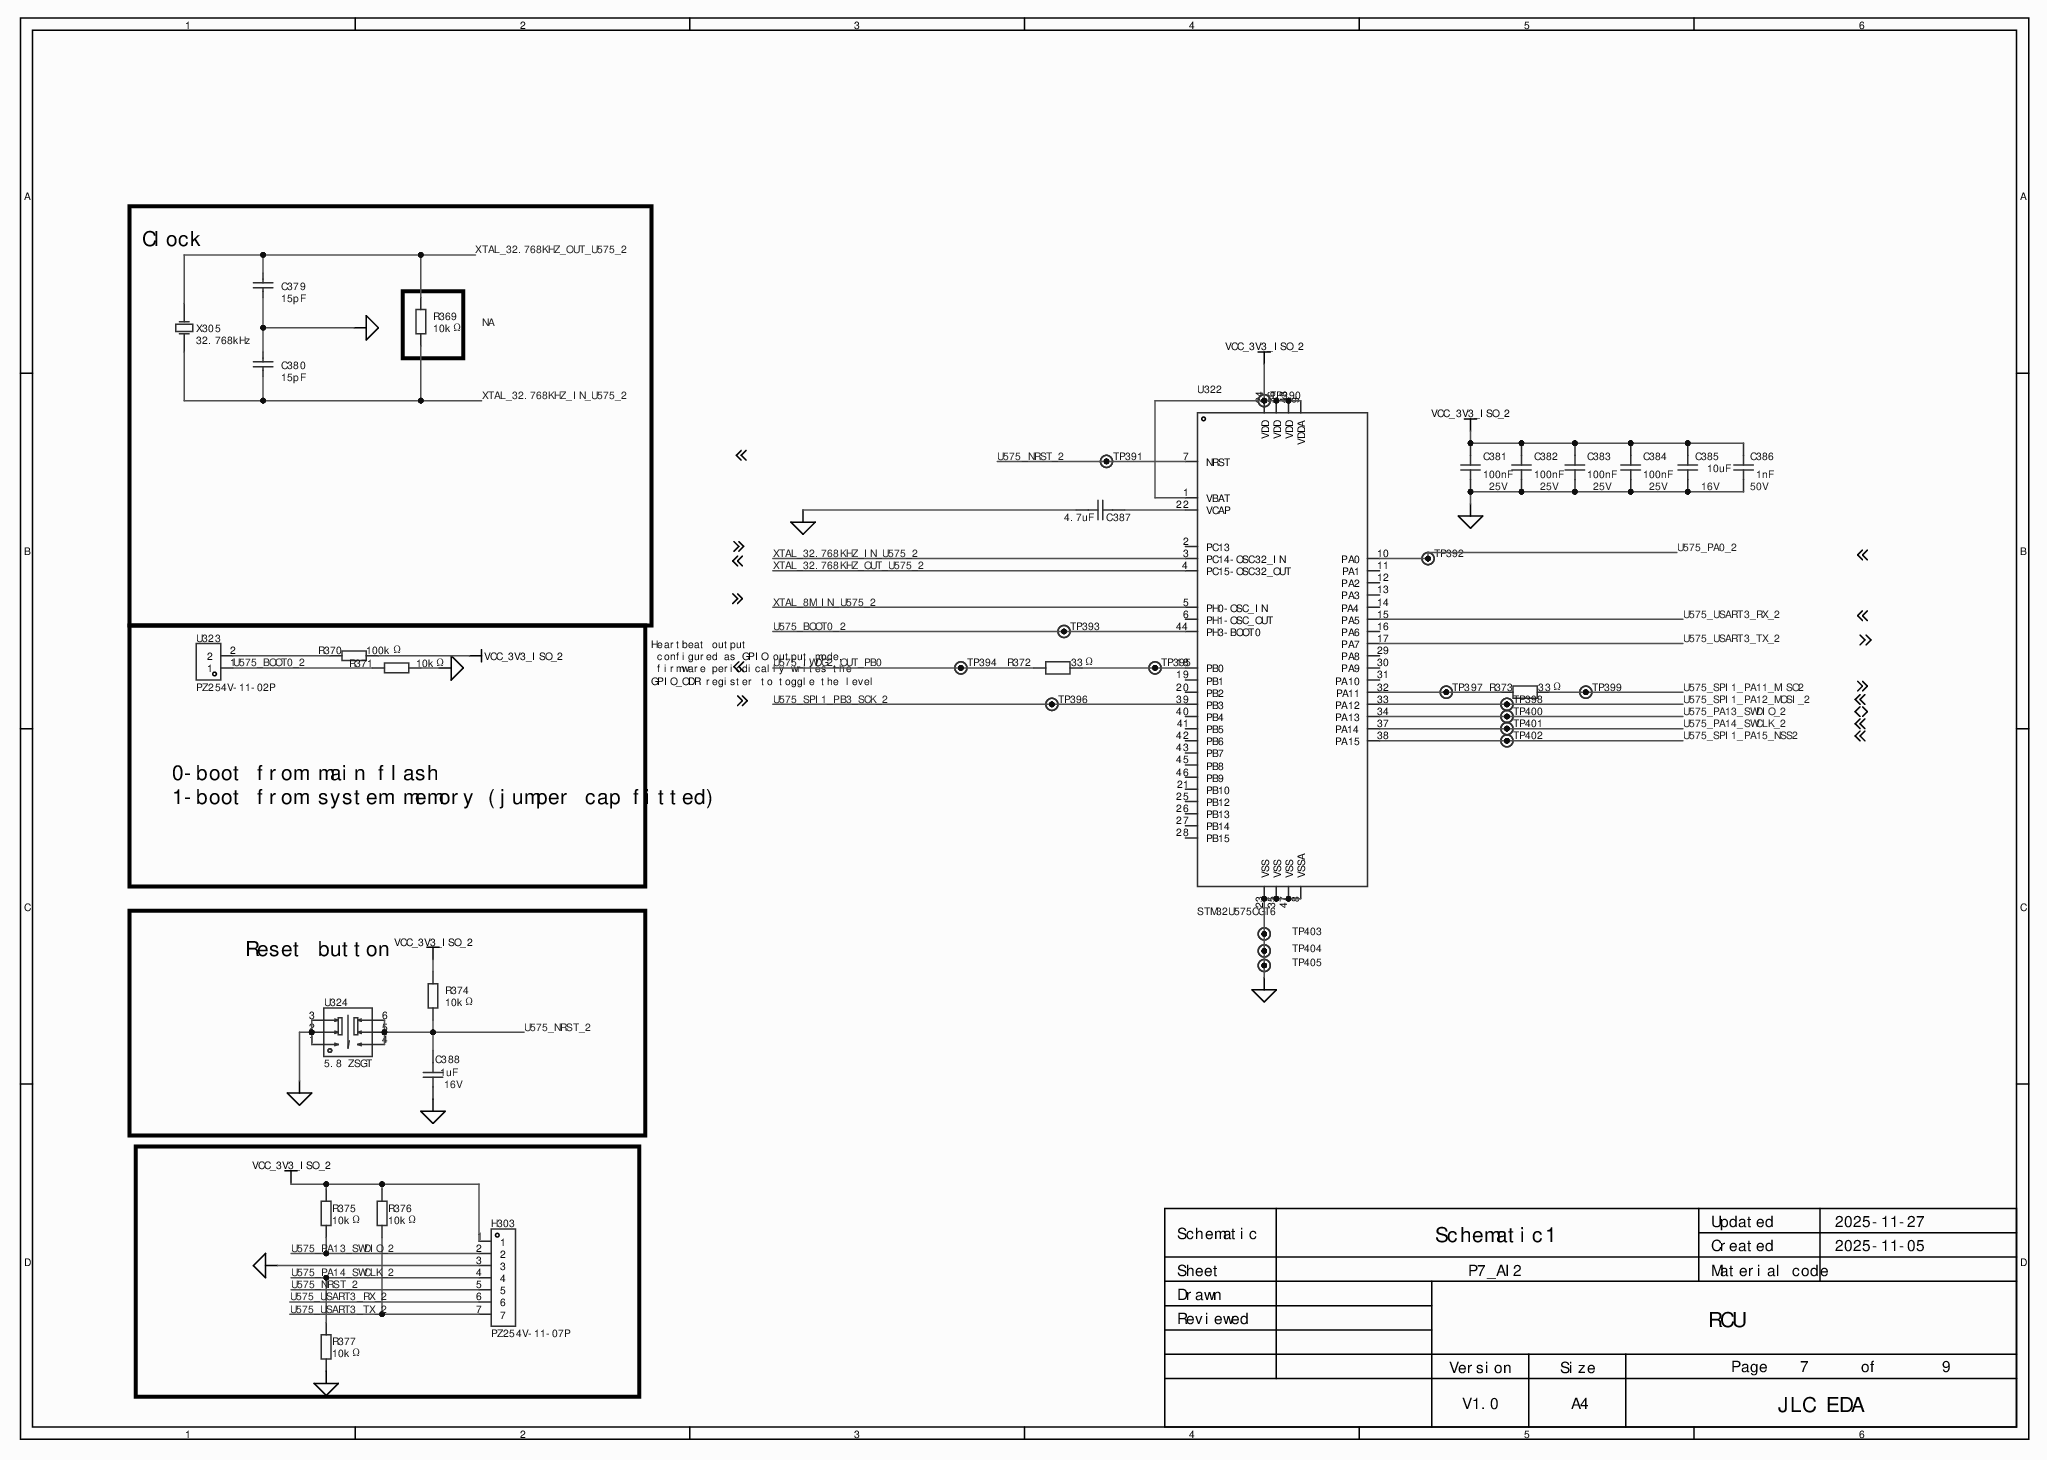
[diagram p0: MISC84429-8.SchDoc]
# Altium project MISC84429-12.PrjPcb (part 4 of 5)

## Sheet MISC84429-8.SchDoc
size 431 x 309 mm; Name: Sheet-Symbol; Symbol: Sheet-Symbol; Device: Sheet-Symbol

### Parts
C379  15pF  [C0402]
C380  15pF  [C0402]
C381  100nF  Voltage Rated: 25V  [C0603]
C382  100nF  Voltage Rated: 25V  [C0603]
C383  100nF  Voltage Rated: 25V  [C0603]
C384  100nF  Voltage Rated: 25V  [C0603]
C385  10uF  Voltage Rated: 16V  [C0805]
C386  1nF  Voltage Rated: 50V  [C0603]
C387  4.7uF  [C0603]
C388  1uF  Voltage Rated: 16V  [C0603]
H303  PZ254V-11-07P  [HDR-TH_7P-P2.54-V-M]
R369  10kΩ  [R0402]
R370  100kΩ  [R0603]
R371  10kΩ  [R0603]
R372  33Ω  [R0603]
R373  33Ω  [R0603]
R374  10kΩ  [R0402]
R375  10kΩ  [R0603]
R376  10kΩ  [R0603]
R377  10kΩ  [R0603]
TP390  (no value)  [Test-Point-0.5mm]
TP391  (no value)  [Test-Point-0.5mm]
TP392  (no value)  [Test-Point-0.5mm]
TP393  (no value)  [Test-Point-0.5mm]
TP394  (no value)  [Test-Point-0.5mm]
TP395  (no value)  [Test-Point-0.5mm]
TP396  (no value)  [Test-Point-0.5mm]
TP397  (no value)  [Test-Point-0.5mm]
TP398  (no value)  [Test-Point-0.5mm]
TP399  (no value)  [Test-Point-0.5mm]
TP400  (no value)  [Test-Point-0.5mm]
TP401  (no value)  [Test-Point-0.5mm]
TP402  (no value)  [Test-Point-0.5mm]
TP403  (no value)  [Test-Point-0.5mm]
TP404  (no value)  [Test-Point-0.5mm]
TP405  (no value)  [Test-Point-0.5mm]
U322  STM32U575CGT6  [LQFP-48_L7.0-W7.0-P0.50-LS9.0-TL]
U323  PZ254V-11-02P  [HDR-TH_2P-P2.54-V-M]
U324  5.8 ZSGT  [SW-TH_5.8ZSGT]
X305  32.768kHz  [OSC-TH_BD3.1-P0.8-D0.3]

### Blocks framed on the sheet
Clock: C379 C380 R369 X305
Reset button: C388 R374 U324

### Nets
PGND: C379.1 C380.2 C381.2 C382.2 C383.2 C384.2 C385.1 C386.1 C387.2 C388.1 H303.3 R371.1 R377.2 TP403.1 TP404.1 TP405.1 U322.8(VSSA) U322.23(VSS) U322.35(VSS) U322.47(VSS) U324.1 U324.2 U324.3
VCC_3V3_ISO_2: C381.1 C382.1 C383.1 C384.1 C385.2 C386.2 H303.1 R370.2 R374.2 R375.2 R376.2 TP390.1 U322.1(VBAT) U322.9(VDDA) U322.24(VDD) U322.36(VDD) U322.48(VDD)
U575_BOOT0_2: R371.2 TP393.1 U322.44(PH3-BOOT0) U323.1
U575_IWDG2_OUT_PB0: R372.2 TP394.1
U575_NRST_2: C388.2 H303.5 R374.1 TP391.1 U322.7(NRST) U324.4 U324.5 U324.6
U575_PA0_2: TP392.1 U322.10(PA0)
U575_PA13_SWDIO_2: H303.2 R375.1 TP400.1 U322.34(PA13)
U575_PA14_SWCLK_2: H303.4 R377.1 TP401.1 U322.37(PA14)
U575_SPI1_PA11_MISO2: R373.1 TP399.1
U575_SPI1_PA12_MOSI_2: TP398.1 U322.33(PA12)
U575_SPI1_PA15_NSS2: TP402.1 U322.38(PA15)
U575_SPI1_PB3_SCK_2: TP396.1 U322.39(PB3)
U575_USART3_RX_2: H303.6 U322.15(PA5)
U575_USART3_TX_2: H303.7 R376.1 U322.17(PA7)
XTAL_8M_IN_U575_2: U322.5(PH0-OSC_IN)
XTAL_32.768KHZ_IN_U575_2: C380.1 R369.1 U322.3(PC14-OSC32_IN) X305.1(OSC1)
XTAL_32.768KHZ_OUT_U575_2: C379.2 R369.2 U322.4(PC15-OSC32_OUT) X305.2(OSC2)
NetC387_1: C387.1 U322.22(VCAP)
NetR370_1: R370.1 U323.2
NetR372_1: R372.1 TP395.1 U322.18(PB0)
NetR373_2: R373.2 TP397.1 U322.32(PA11)

Not connected (* = marked no-connect by the designer): U322 2(PC13)* 6(PH1-OSC_OUT)* 11(PA1)* 12(PA2)* 13(PA3)* 14(PA4)* 16(PA6)* 19(PB1)* 20(PB2)* 21(PB10)* 25(PB12)* 26(PB13)* 27(PB14)* 28(PB15)* 29(PA8)* 30(PA9)* 31(PA10)* 40(PB4)* 41(PB5)* 42(PB6)* 43(PB7)* 45(PB8)* 46(PB9)*

### Notes on the sheet
- NA
- Heartbeat output
  configured as GPIO output mode,
  firmware periodically writes the
  GPIO_ODR register to toggle the level
- 0-boot from main flash
  1-boot from system memory (jumper cap fitted)
- 1
- 2
- 3
- 4
- 5
- 6
- A
- B
- C
- D
- Schematic
- Schematic1
- Created
- Updated
- 2025-11-27
- 2025-11-05
- Reviewed
- Drawn
- Sheet
- P7_AI2
- Material code
- RCU
- Version
- Size
- Page
- 7
- of
- 9
- V1.0
- A4
- JLC EDA

### Library data of the parts
C379 C380 = GJM1555C1H150FB01D: Manufacturer: muRata(村田); Add into BOM: yes; Tolerance: ±1%; Voltage Rated: 50V; Temperature Coefficient: C0G; Symbol: GJM1555C1H150FB01D; Device: GJM1555C1H150FB01D; LCSC Part Name: 15pF ±1% 50V; Supplier Part: C441742; Manufacturer Part: GJM1555C1H150FB01D; Supplier Footprint: 0402; JLCPCB Part Class: Extended library; Datasheet: https://atta.szlcsc.com/upload/public/pdf/source/20200305/C490387_23319AE8C154DEB24C505E6C82A8106A.pdf; Supplier: LCSC; Convert to PCB: yes; Value: 15pF; Origin Footprint: C0402
C381-C384 = GRM188R71E104KA01D: Manufacturer: muRata(村田); Add into BOM: yes; Tolerance: ±10%; Temperature Coefficient: X7R; Symbol: GRM188R71E104KA01D; Device: GRM188R71E104KA01D; LCSC Part Name: 100nF ±10% 25V; Supplier Part: C77050; Manufacturer Part: GRM188R71E104KA01D; Supplier Footprint: 0603; JLCPCB Part Class: Extended library; Datasheet: https://atta.szlcsc.com/upload/public/pdf/source/20170622/1498103881034.pdf; Supplier: LCSC; Convert to PCB: yes; Value: 100nF; Origin Footprint: C0603
C385 = GRM21BR61C106KE15L: Manufacturer: muRata(村田); Add into BOM: yes; Tolerance: ±10%; Temperature Coefficient: X5R; Symbol: GRM21BR61C106KE15L; Device: GRM21BR61C106KE15L; LCSC Part Name: 10uF ±10% 16V; Supplier Part: C77075; Manufacturer Part: GRM21BR61C106KE15L; Supplier Footprint: 0805; JLCPCB Part Class: Extended library; Datasheet: https://atta.szlcsc.com/upload/public/pdf/source/20200305/C490387_23319AE8C154DEB24C505E6C82A8106A.pdf; Supplier: LCSC; Convert to PCB: yes; Value: 10uF; Origin Footprint: C0805
C386 = GRM1885C1H102JA01D: Manufacturer: muRata(村田); Add into BOM: yes; Tolerance: ±5%; Temperature Coefficient: C0G; Symbol: GRM1885C1H102JA01D; Device: GRM1885C1H102JA01D; LCSC Part Name: 1nF ±5% 50V; Supplier Part: C77026; Manufacturer Part: GRM1885C1H102JA01D; Supplier Footprint: 0603; JLCPCB Part Class: Extended library; Datasheet: https://atta.szlcsc.com/upload/public/pdf/source/20200305/C490387_23319AE8C154DEB24C505E6C82A8106A.pdf; Supplier: LCSC; Convert to PCB: yes; Value: 1nF; Origin Footprint: C0603
C387 = GRT188C81E475KE13D: Manufacturer: muRata(村田); Add into BOM: yes; Tolerance: ±10%; Voltage Rating: 25V; Temperature Coefficient: X6S; Symbol: GRT188C81E475KE13D; Device: GRT188C81E475KE13D; LCSC Part Name: 4.7uF ±10% 25V; Supplier Part: C907917; Manufacturer Part: GRT188C81E475KE13D; Supplier Footprint: 0603; JLCPCB Part Class: Extended library; Datasheet: https://item.szlcsc.com/datasheet/GRT188C81E475KE13D/973818.html; Supplier: LCSC; Convert to PCB: yes; Value: 4.7uF; Origin Footprint: C0603
C388 = GCM188R71C105KA64D: Manufacturer: muRata(村田); Add into BOM: yes; Tolerance: ±10%; Temperature Coefficient: X7R; Symbol: GCM188R71C105KA64D; Device: GCM188R71C105KA64D; LCSC Part Name: 1uF ±10% 16V; Supplier Part: C161212; Manufacturer Part: GCM188R71C105KA64D; Supplier Footprint: 0603; JLCPCB Part Class: Extended library; Datasheet: https://atta.szlcsc.com/upload/public/pdf/source/20181221/C161212_C96DD77354D5551432B3B7779E4D1948.pdf; Supplier: LCSC; Convert to PCB: yes; Value: 1uF; Origin Footprint: C0603
H303 = PZ254V-11-07P: Manufacturer: XFCN(兴飞); Add into BOM: yes; Pin Structure: 1x7P; Pitch: 2.54mm; Circluar Pins/Square Pins: Square pin; Symbol: PZ254V-11-07P; Device: PZ254V-11-07P; LCSC Part Name: 1x7P 间距:2.54mm 方针 直插; Supplier Part: C492406; Manufacturer Part: PZ254V-11-07P; Supplier Footprint: 插件,P=2.54mm; JLCPCB Part Class: Extended library; Datasheet: https://atta.szlcsc.com/upload/public/pdf/source/20200309/C492406_654C533EE691117E22DD9F76C114C2D9.pdf; Supplier: LCSC; Convert to PCB: yes; Row Spacing: -; Mounting Type: Through hole; Number of Rows: Single row; Number of Pins: 7P; Current Rating: -; Voltage Rating (Max): -; Length of Mating Pin: 6mm; Insulation Height: 2.5mm; Length of End Connection Pin: 3mm; Contact Material: Brass; Contact Plating: -; Operating Temperature: -40℃~+105℃; Color: Black; Origin Footprint: HDR-TH_7P-P2.54-V-M
R369 R374 = 0402WGF1002TCE: Manufacturer: UNI-ROYAL(厚声); Add into BOM: yes; Tolerance: ±1%; Power(Watts): 62.5mW; Overload Voltage (Max): 50V; Temperature Coefficient: ±100ppm/℃; Symbol: 0402WGF1002TCE; Device: 0402WGF1002TCE; LCSC Part Name: 10kΩ ±1% 62.5mW 厚膜电阻; Supplier Part: C25744; Manufacturer Part: 0402WGF1002TCE; Supplier Footprint: 0402; JLCPCB Part Class: Basic library; Datasheet: https://atta.szlcsc.com/upload/public/pdf/source/20200306/C422600_1E6D84923E4A46A82E41ADD87F860B5C.pdf; Supplier: LCSC; Convert to PCB: yes; Type: Thick film resistor; Value: 10kΩ; Operating Temperature Range: -55℃~+155℃; Origin Footprint: R0402
R370 = RC0603FR-07100KL: Manufacturer: YAGEO(国巨); Add into BOM: yes; Tolerance: ±1%; Power(Watts): 100mW; Overload Voltage (Max): 75V; Temperature Coefficient: ±100ppm/℃; Symbol: RC0603FR-07100KL; Device: RC0603FR-07100KL; LCSC Part Name: 厚膜电阻 100kΩ ±1% 100mW; Supplier Part: C14675; Manufacturer Part: RC0603FR-07100KL; Supplier Footprint: 0603; JLCPCB Part Class: Extended library; Datasheet: https://atta.szlcsc.com/upload/public/pdf/source/20140324/1457707028752.pdf; Supplier: LCSC; Convert to PCB: yes; Type: Thick film resistor; Value: 100kΩ; Operating Temperature Range: -55℃~+155℃; Origin Footprint: R0603
R371 R375-R377 = RC0603FR-0710KL: Manufacturer: YAGEO(国巨); Add into BOM: yes; Tolerance: ±1%; Power(Watts): 100mW; Overload Voltage (Max): 75V; Temperature Coefficient: ±100ppm/℃; Symbol: RC0603FR-0710KL; Device: RC0603FR-0710KL; LCSC Part Name: 厚膜电阻 10kΩ ±1% 100mW; Supplier Part: C98220; Manufacturer Part: RC0603FR-0710KL; Supplier Footprint: 0603; JLCPCB Part Class: Extended library; Datasheet: https://atta.szlcsc.com/upload/public/pdf/source/20180927/C295883_E8D83085EA81BD7DE0B2B681138C15EE.pdf; Supplier: LCSC; Convert to PCB: yes; Type: Thick film resistor; Value: 10kΩ; Operating Temperature Range: -55℃~+155℃; Origin Footprint: R0603
R372 R373 = FRC0603F33R0TS: Manufacturer: FOJAN(富捷); Add into BOM: yes; Tolerance: ±1%; Power(Watts): 100mW; Voltage-Supply(Max): 75V; Temperature Coefficient: ±100ppm/℃; Symbol: FRC0603F33R0TS; Device: FRC0603F33R0TS; LCSC Part Name: 33Ω ±1% 100mW 厚膜电阻; Supplier Part: C2909394; Manufacturer Part: FRC0603F33R0TS; Supplier Footprint: 0603; JLCPCB Part Class: Extended library; Supplier: LCSC; Convert to PCB: yes; Type: Thick film resistor; Value: 33Ω; Operating Temperature: -55℃~+155℃; Origin Footprint: R0603
TP390-TP405 = Test-Point: Add into BOM: yes; Symbol: Test-Point; Device: Test-Point; Convert to PCB: yes; Origin Footprint: Test-Point-0.5mm
U322 = STM32U575CGT6: Manufacturer: ST(意法半导体); Add into BOM: yes; Symbol: STM32U575CGT6; Device: STM32U575CGT6; LCSC Part Name: 超低功耗带 FPU 的 Arm Cortex-M33 具有 Trust Zone，160 MHz MCU 带 1MB 闪存; Supplier Part: C5271006; Manufacturer Part: STM32U575CGT6; Supplier Footprint: LQFP-48(7x7); JLCPCB Part Class: Extended library; Datasheet: https://atta.szlcsc.com/upload/public/pdf/source/20250311/118E46867C2F8A0EF1AEA9206C957AC0.pdf; Supplier: LCSC; Convert to PCB: yes; Origin Footprint: LQFP-48_L7.0-W7.0-P0.50-LS9.0-TL
U323 = PZ254V-11-02P: Manufacturer: XFCN(兴飞); Add into BOM: yes; Pin Structure: 1x2P; Pitch: 2.54mm; Circluar Pins/Square Pins: Square pin; Symbol: PZ254V-11-02P; Device: PZ254V-11-02P; LCSC Part Name: 间距:2.54mm 1x2P 直插 方针; Supplier Part: C492401; Manufacturer Part: PZ254V-11-02P; Supplier Footprint: 插件,P=2.54mm; JLCPCB Part Class: Extended library; Datasheet: https://atta.szlcsc.com/upload/public/pdf/source/20200309/C492401_A812433581A9B211A7FFA413ADDFF0E5.pdf; Supplier: LCSC; Convert to PCB: yes; Row Spacing: -; Mounting Type: Through hole; Number of Rows: Single row; Number of Pins: 2P; Current Rating (Max): -; Voltage Rating (Max): -; Length of Mating Pin: 6mm; Insulation Height: 2.5mm; Length of End Connection Pin: 3mm; Contact Material: Brass; Contact Plating: -; Operating Temperature Range: -40℃~+105℃; Color: Black; Origin Footprint: HDR-TH_2P-P2.54-V-M
U324 = 5.8 ZSGT: Manufacturer: SHOU HAN(首韩); Add into BOM: yes; Circuit: DPDT; Self Lock / No Lock: Self-locking; Actuator Style: Square button; Contact Current: 110mA; Voltage Rating (DC): 30V; Insulation Resistance: 100MΩ; Actuator/Cap Color: White; With Lamp: Without; Pin Style: PC pin; Operating Force: 1.5N; Mechanical Life: 10 ten-thousand cycles; Symbol: 5.8 ZSGT; Device: 5.8 ZSGT; LCSC Part Name: 5.8*5.8有头/高头 带锁/自锁开关 泡泡机开关; Supplier Part: C2681587; Manufacturer Part: 5.8 ZSGT; Supplier Footprint: 插件; JLCPCB Part Class: Extended library; Datasheet: https://atta.szlcsc.com/upload/public/pdf/source/20210107/C2681587_CDDDDA4A1C7AC9FEB01815B75893A6BA.pdf; Supplier: LCSC; Convert to PCB: yes; Mounting Style: Through hole; Operating Temperature: -10℃~+70℃; Origin Footprint: SW-TH_5.8ZSGT
X305 = X308032768KGB2SC: Manufacturer: YXC(扬兴晶振); Add into BOM: yes; Normal temperature Frequency Tolerance: ±10ppm; Load Capacitance: 12.5pF; Frequency Stability: ±20ppm; Symbol: X308032768KGB2SC; Device: X308032768KGB2SC; LCSC Part Name: YT-38 32.768KHZ 2P 3080 12.5PF ±10PPM -20~70℃; Supplier Part: C52082; Manufacturer Part: X308032768KGB2SC; Supplier Footprint: DT-38; JLCPCB Part Class: Extended library; Datasheet: https://item.szlcsc.com/datasheet/X308032768KGB2SC/53096.html; Supplier: LCSC; Convert to PCB: yes; Type: Through-hole crystal; Value: 32.768kHz; Operating Temperature: -20℃~+70℃; Origin Footprint: OSC-TH_BD3.1-P0.8-D0.3

## Sheet MISC84429-10.SchDoc
size 309 x 223 mm; Name: Sheet-Symbol; Symbol: Sheet-Symbol; Device: Sheet-Symbol
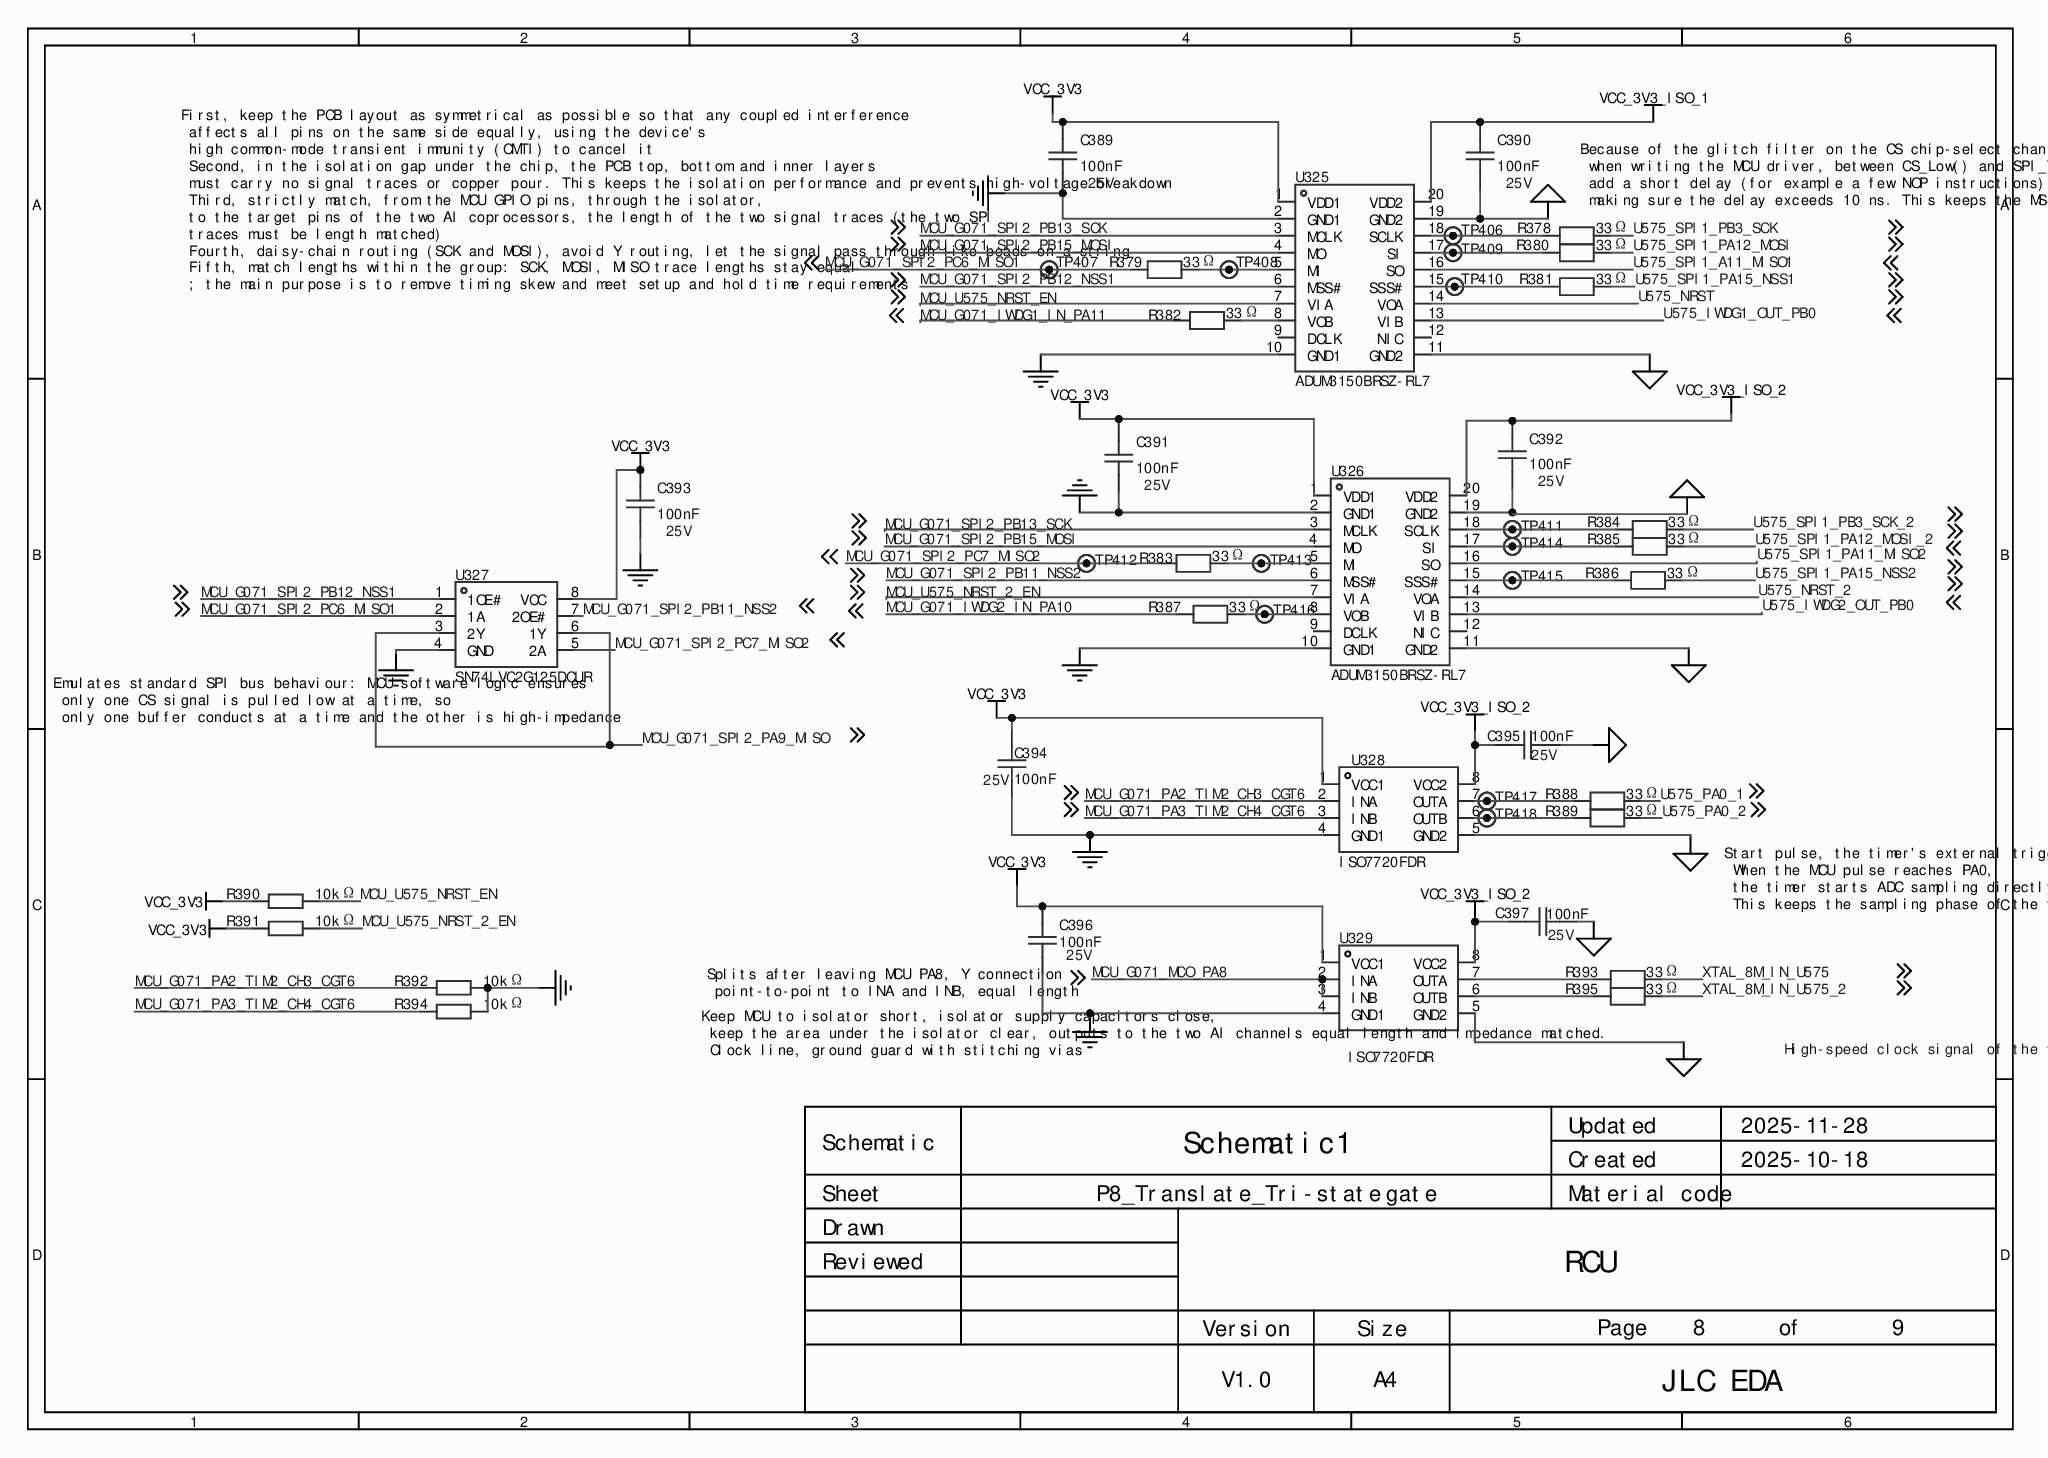
[diagram p1: MISC84429-10.SchDoc]

### Parts
C389  100nF  Voltage Rated: 25V  [C0603]
C390  100nF  Voltage Rated: 25V  [C0603]
C391  100nF  Voltage Rated: 25V  [C0603]
C392  100nF  Voltage Rated: 25V  [C0603]
C393  100nF  Voltage Rated: 25V  [C0603]
C394  100nF  Voltage Rated: 25V  [C0603]
C395  100nF  Voltage Rated: 25V  [C0603]
C396  100nF  Voltage Rated: 25V  [C0603]
C397  100nF  Voltage Rated: 25V  [C0603]
R378  33Ω  [R0603]
R379  33Ω  [R0603]
R380  33Ω  [R0603]
R381  33Ω  [R0603]
R382  33Ω  [R0603]
R383  33Ω  [R0603]
R384  33Ω  [R0603]
R385  33Ω  [R0603]
R386  33Ω  [R0603]
R387  33Ω  [R0603]
R388  33Ω  [R0603]
R389  33Ω  [R0603]
R390  10kΩ  [R0603]
R391  10kΩ  [R0603]
R392  10kΩ  [R0603]
R393  33Ω  [R0603]
R394  10kΩ  [R0603]
R395  33Ω  [R0603]
TP406  (no value)  [Test-Point-0.5mm]
TP407  (no value)  [Test-Point-0.5mm]
TP408  (no value)  [Test-Point-0.5mm]
TP409  (no value)  [Test-Point-0.5mm]
TP410  (no value)  [Test-Point-0.5mm]
TP411  (no value)  [Test-Point-0.5mm]
TP412  (no value)  [Test-Point-0.5mm]
TP413  (no value)  [Test-Point-0.5mm]
TP414  (no value)  [Test-Point-0.5mm]
TP415  (no value)  [Test-Point-0.5mm]
TP416  (no value)  [Test-Point-0.5mm]
TP417  (no value)  [Test-Point-0.5mm]
TP418  (no value)  [Test-Point-0.5mm]
U325  ADUM3150BRSZ-RL7  [SSOP-20_L7.2-W5.3-P0.65-LS7.8-BL]
U326  ADUM3150BRSZ-RL7  [SSOP-20_L7.2-W5.3-P0.65-LS7.8-BL]
U327  SN74LVC2G125DCUR  [VSON8_L2.0-W2.3-P0.50-LS3.1-BL]
U328  ISO7720FDR  [SOIC-8_L5.0-W4.0-P1.27-LS6.1-BL]
U329  ISO7720FDR  [SOIC-8_L5.0-W4.0-P1.27-LS6.1-BL]

### Nets
GND: C389.2 C391.2 C393.2 C394.2 C396.2 R392.2 R394.2 U325.2(GND1) U325.10(GND1) U326.2(GND1) U326.10(GND1) U327.4(GND) U328.4(GND1) U329.4(GND1)
PGND: C390.2 C392.2 C395.2 C397.2 U325.11(GND2) U325.19(GND2) U326.11(GND2) U326.19(GND2) U328.5(GND2) U329.5(GND2)
VCC_3V3: C389.1 C391.1 C393.1 C394.1 C396.1 R390.1 R391.1 U325.1(VDD1) U326.1(VDD1) U327.8(VCC) U328.1(VCC1) U329.1(VCC1)
VCC_3V3_ISO_1: C390.1 U325.20(VDD2)
VCC_3V3_ISO_2: C392.1 C395.1 C397.1 U326.20(VDD2) U328.8(VCC2) U329.8(VCC2)
MCU_G071_IWDG1_IN_PA11: R382.2
MCU_G071_IWDG2_IN_PA10: R387.2
MCU_G071_MCO_PA8: U329.2(INA) U329.3(INB)
MCU_G071_PA2_TIM2_CH3_CGT6: R392.1 U328.2(INA)
MCU_G071_PA3_TIM2_CH4_CGT6: R394.1 U328.3(INB)
MCU_G071_SPI2_PA9_MISO: U327.3(2Y) U327.6(1Y)
MCU_G071_SPI2_PB11_NSS2: U326.6(MSS#) U327.7(2OE#)
MCU_G071_SPI2_PB12_NSS1: U325.6(MSS#) U327.1(1OE#)
MCU_G071_SPI2_PB13_SCK: U325.3(MCLK) U326.3(MCLK)
MCU_G071_SPI2_PB15_MOSI: U325.4(MO) U326.4(MO)
MCU_G071_SPI2_PC6_MISO1: R379.2 TP407.1 U327.2(1A)
MCU_G071_SPI2_PC7_MISO2: R383.2 TP412.1 U327.5(2A)
MCU_U575_NRST_2_EN: R391.2 U326.7(VIA)
MCU_U575_NRST_EN: R390.2 U325.7(VIA)
U575_IWDG1_OUT_PB0: U325.13(VIB)
U575_IWDG2_OUT_PB0: U326.13(VIB)
U575_NRST: U325.14(VOA)
U575_NRST_2: U326.14(VOA)